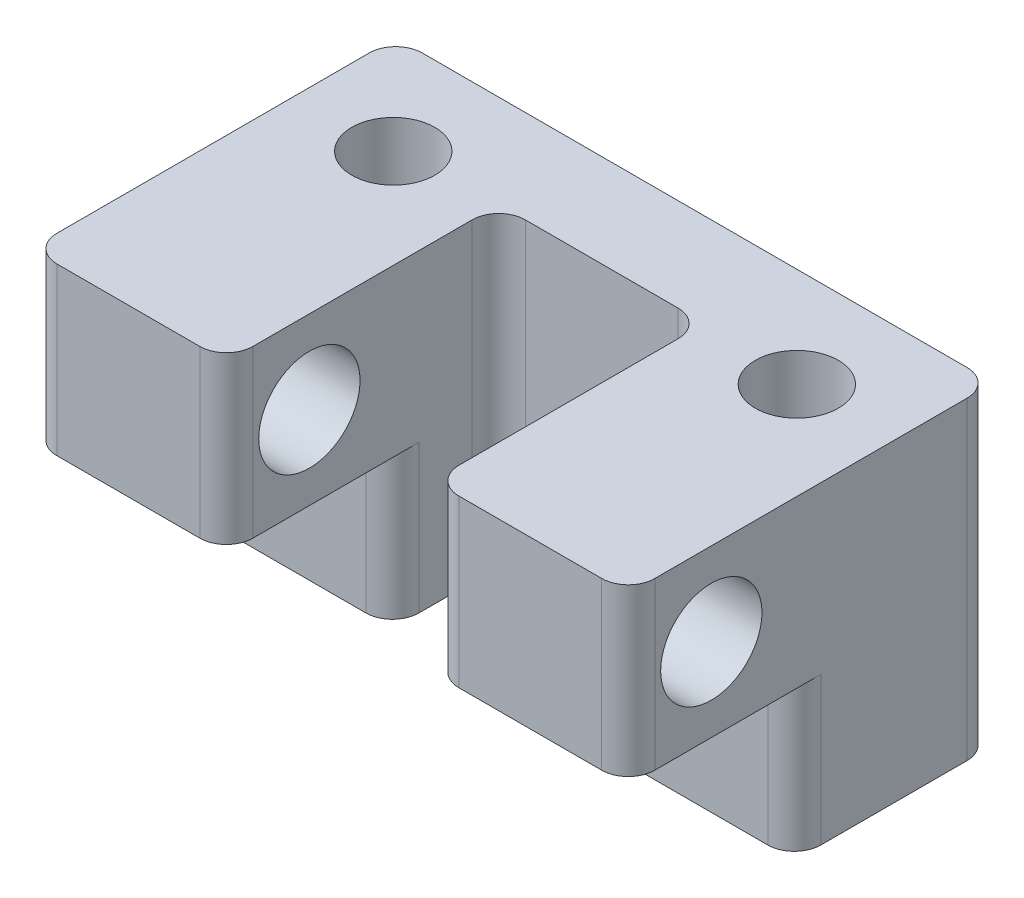
SolidWorks part; units mm, degrees
material "6061 合金"
ref_plane "前视基准面" through (0, 0, 0) normal (0, 0, 1) x (1, 0, 0)
ref_plane "上视基准面" through (0, 0, 0) normal (0, 1, 0) x (1, 0, 0)
ref_plane "右视基准面" through (0, 0, 0) normal (1, 0, 0) x (0, 0, -1)
sketch "草图1" plane through (0, 0, 0) normal (0, 1, 0) x (1, 0, 0)
  line L0 (-9, 2.8) -> (9, 2.8)
  line L5 (9, 2.8) -> (9, -3.2)
  line L6 (9, -3.2) -> (3.1, -3.2)
  line L7 (3.1, -3.2) -> (3.1, 0)
  line L8 (3.1, 0) -> (-3.1, 0)
  line L9 (-3.1, 0) -> (-3.1, -3.2)
  line L10 (-3.1, -3.2) -> (-9, -3.2)
  line L11 (-9, -3.2) -> (-9, 2.8)
  line L12 (0, 2.8) -> (0, 0) construction
  point P0 (0, 0)
  dimension "D1" = 6
  dimension "D4" = 5.9
  dimension "D2" = 18
  dimension "D3" = 3.2
extrude "凸台-拉伸1" add sketch "草图1" along normal blind 4.45
sketch "草图2" plane through (0, 4.45, 0) normal (0, 1, 0) x (1, 0, 0)
  line L0 (-3.1, -3.2) -> (-3.1, 0) construction
  line L1 (-3.1, 0) -> (3.1, 0) construction
  line L2 (3.1, 0) -> (3.1, -3.2) construction
  line L3 (9, -3.2) -> (9, 2.8) construction
  line L4 (9, 2.8) -> (-9, 2.8) construction
  line L5 (-9, 2.8) -> (-9, -3.2) construction
  line L6 (-3.1, -8.2) -> (-3.1, 0)
  line L7 (-3.1, 0) -> (3.1, 0)
  line L8 (3.1, 0) -> (3.1, -8.2)
  line L9 (9, -8.2) -> (9, 2.8)
  line L10 (9, 2.8) -> (-9, 2.8)
  line L11 (-9, 2.8) -> (-9, -8.2)
  line L12 (-9, -8.2) -> (-3.1, -8.2)
  line L13 (3.1, -8.2) -> (9, -8.2)
  line L14 (-9, -3.2) -> (-3.1, -3.2) construction
  dimension "D1" = 5
extrude "凸台-拉伸2" add sketch "草图2" along normal blind 5
sketch "草图3" plane through (0, 0, 0) normal (0, -1, 0) x (1, 0, 0)
  line L0 (0, 0) -> (0, -2.8) construction
  line L1 (9, -2.8) -> (-9, -2.8) construction
  point P0 (-6.075, 0.2)
  point P1 (6.075, 0.2)
  point P13 (-15.7826, 3.935)
  dimension "D1" = 12.15
  dimension "D2" = 3
hole_wizard "M3 螺纹孔1" positions "草图3" profile "草图4" tap size "M3" standard "GB" end condition through all
sketch "草图4" plane through (-6.075, 0, 0.2) normal (1, 0, 0) x (0, 0, -1)
  line L0 (0, 0) -> (0, 9.45)
  line L1 (0, 9.45) -> (1.25, 9.45)
  line L2 (1.25, 9.45) -> (1.25, 0)
  line L5 (1.25, 0) -> (0, 0)
  line L11 (0, -6.35) -> (0, 107.95) construction
  dimension "通孔螺纹孔钻头直径" = 2.5
  dimension "通孔螺纹孔钻头深度" = 9.45
cosmetic thread "孔螺纹线1" parameters "D2"=3
cosmetic thread "孔螺纹线2" parameters "D2"=3
sketch "草图5" plane through (-9, 0, 0) normal (-1, 0, 0) x (0, 0, 1)
  line L0 (8.2, 9.45) -> (8.2, 4.45) construction
  line L1 (-2.8, 9.45) -> (8.2, 9.45) construction
  circle A0 centre (5.7, 6.95) radius 1.525
  dimension "D1" = 3.05
  dimension "D2" = 2.5
  dimension "D3" = 2.5
extrude "切除-拉伸1" cut sketch "草图5" against normal through all
fillet "R0.8 圆角1" radius 0.8 12 edges at (3.1, 4.725, 0) (-3.1, 4.725, 0) (-9, 4.725, -2.8) (9, 4.725, -2.8) (9, 6.95, 8.2) (3.1, 6.95, 8.2) (-3.1, 6.95, 8.2) (-9, 6.95, 8.2) (-9, 2.225, 3.2) (-3.1, 2.225, 3.2) (3.1, 2.225, 3.2) (9, 2.225, 3.2)
